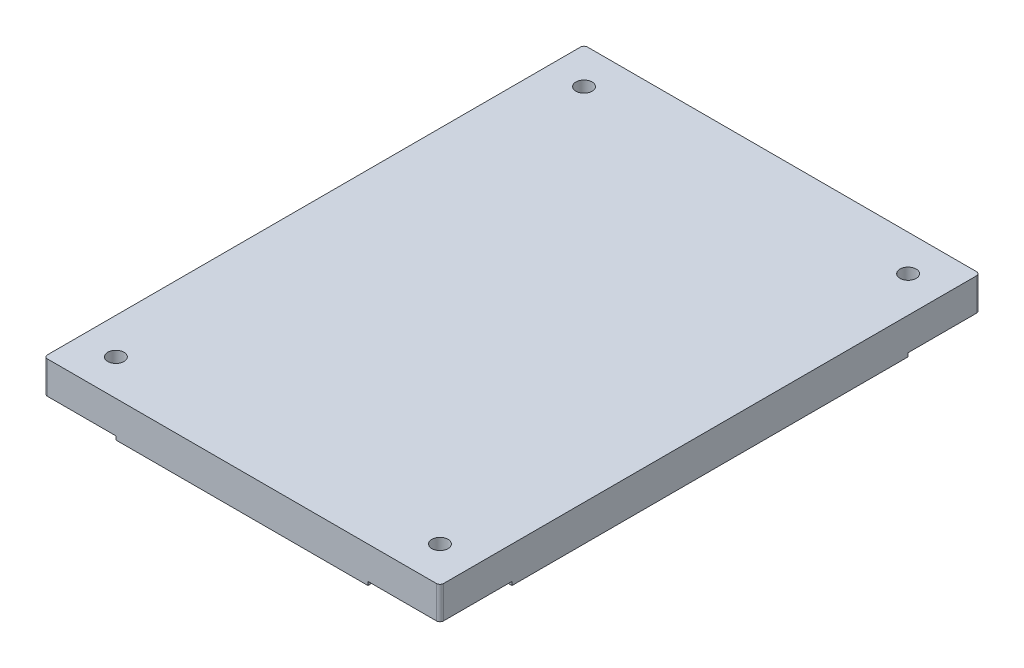
from build123d import *

# Parameters (mm, degrees)
SKETCH1_W                  = 110
SKETCH1_H                  = 150
BOSS_EXTRUDE1_DEPTH        = 10
SKETCH2_W                  = 20
SKETCH2_H                  = 20
CUT_EXTRUDE1_DEPTH         = 1
F_4_5_4_5_DIAMETER_HOLE1_D = 4.5
FILLET1_R                  = 1
FILLET2_R                  = 1


with BuildPart() as part:
    # Sketch1 → Boss-Extrude1 (new body)
    with BuildSketch(Plane(origin=(0, 0, 0), x_dir=(1, 0, 0), z_dir=(0, 1, 0))):
        Rectangle(SKETCH1_W, SKETCH1_H)
    extrude(amount=BOSS_EXTRUDE1_DEPTH)

    # Sketch2 → Cut-Extrude1 (cut)
    with BuildSketch(Plane.XZ):
        with Locations((-45, 65)):
            Rectangle(SKETCH2_W, SKETCH2_H)
        with Locations((45, 65)):
            Rectangle(SKETCH2_W, SKETCH2_H)
        with Locations((45, -65)):
            Rectangle(SKETCH2_W, SKETCH2_H)
        with Locations((-45, -65)):
            Rectangle(SKETCH2_W, SKETCH2_H)
    extrude(amount=-CUT_EXTRUDE1_DEPTH, mode=Mode.SUBTRACT)

    # Ø4.5 (4.5) Diameter Hole1 (through all)
    with Locations(Plane(origin=(0, 1, 0), x_dir=(-1, 0, 0), z_dir=(0, -1, 0))):
        with Locations((-45, 65), (45, 65), (45, -65), (-45, -65)):
            Hole(F_4_5_4_5_DIAMETER_HOLE1_D / 2)

    # Fillet1
    fillet1_edges = [part.edges().sort_by_distance(p)[0] for p in [
        (-35, 0.5, -55),
        (35, 0.5, -55),
        (35, 0.5, 55),
        (-35, 0.5, 55),
    ]]
    fillet(fillet1_edges, radius=FILLET1_R)

    # Fillet2
    fillet2_edges = [part.edges().sort_by_distance(p)[0] for p in [
        (-55, 5.5, -75),
        (-55, 5.5, 75),
        (55, 5.5, 75),
        (55, 5.5, -75),
    ]]
    fillet(fillet2_edges, radius=FILLET2_R)


solid = part.part
